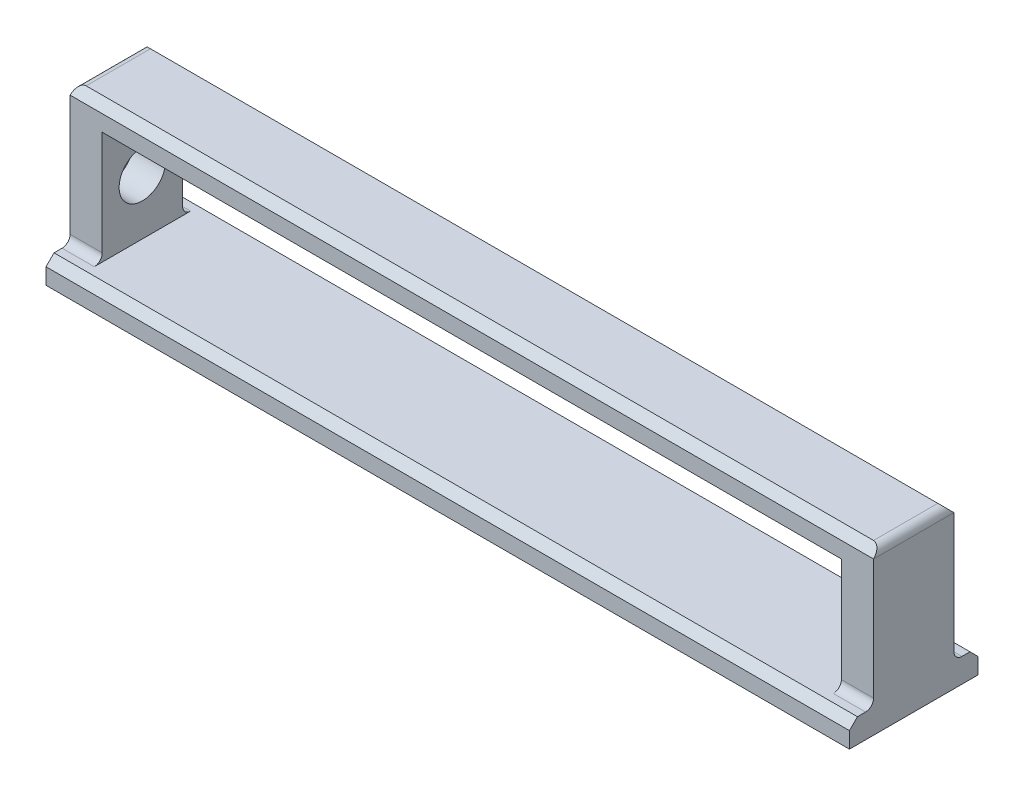
from build123d import *

# Parameters (mm, degrees)
SKETCH1_W               = 5000
SKETCH1_H               = 1000
BOSS_EXTRUDE1_DEPTH     = 250
SKETCH2_W               = 4600
SKETCH2_H               = 700
CUT_EXTRUDE1_DEPTH      = 5124.47538298
CUT_EXTRUDE2_DEPTH      = 5106.144464166
CUT_EXTRUDE2_DEPTH_BACK = 200
SKETCH3_R               = 145
SKETCH4_W               = 5000
SKETCH4_H               = 800
BOSS_EXTRUDE2_DEPTH     = 150
CHAMFER1_SIZE           = 50
FILLET1_R               = 50
FILLET2_R               = 50
SKETCH6_R               = 150
CUT_EXTRUDE3_DEPTH      = 90


with BuildPart() as part:
    # Sketch1 → Boss-Extrude1 (new, symmetric)
    with BuildSketch(Plane.XY):
        with Locations((2500, 500)):
            Rectangle(SKETCH1_W, SKETCH1_H)
    extrude(amount=BOSS_EXTRUDE1_DEPTH, both=True)

    # Sketch2 → Cut-Extrude1 (cut, through all)
    with BuildSketch(Plane.XY.offset(250)):
        with Locations((2500, 500)):
            Rectangle(SKETCH2_W, SKETCH2_H)
    extrude(amount=-CUT_EXTRUDE1_DEPTH, mode=Mode.SUBTRACT)

    # Sketch3 → Cut-Extrude2 (cut, two sides: drawn at the far end of the back side and taken through both)
    with BuildSketch(Plane.ZY.offset(-CUT_EXTRUDE2_DEPTH_BACK)):
        with Locations((0, 500)):
            Circle(SKETCH3_R)
    extrude(amount=CUT_EXTRUDE2_DEPTH + CUT_EXTRUDE2_DEPTH_BACK, mode=Mode.SUBTRACT)

    # Sketch4 → Boss-Extrude2 (add)
    with BuildSketch(Plane.XZ):
        with Locations((2500, 0)):
            Rectangle(SKETCH4_W, SKETCH4_H)
    extrude(amount=-BOSS_EXTRUDE2_DEPTH)

    # Chamfer1
    chamfer1_edges = [part.edges().sort_by_distance(p)[0] for p in [
        (2500, 150, 400),
        (2500, 150, -400),
        (2500, 1000, -250),
        (2500, 1000, 250),
    ]]
    chamfer(chamfer1_edges, length=CHAMFER1_SIZE)

    # Fillet1
    fillet1_edges = [part.edges().sort_by_distance(p)[0] for p in [
        (4900, 150, 250),
        (100, 150, 250),
        (4900, 150, -250),
        (100, 150, -250),
    ]]
    fillet(fillet1_edges, radius=FILLET1_R)

    # Fillet2
    fillet2_edges = [part.edges().sort_by_distance(p)[0] for p in [
        (5000, 1000, 0),
        (0, 1000, 0),
    ]]
    fillet(fillet2_edges, radius=FILLET2_R)

    # Sketch6 → Cut-Extrude3 (cut)
    with BuildSketch(Plane(origin=(4800, 0, 0), x_dir=(0, 0, -1), z_dir=(1, 0, 0))):
        with Locations(Location((0, 500, 0), (0, 0, 180))):
            Circle(SKETCH6_R)
    extrude(amount=CUT_EXTRUDE3_DEPTH, mode=Mode.SUBTRACT)


solid = part.part
